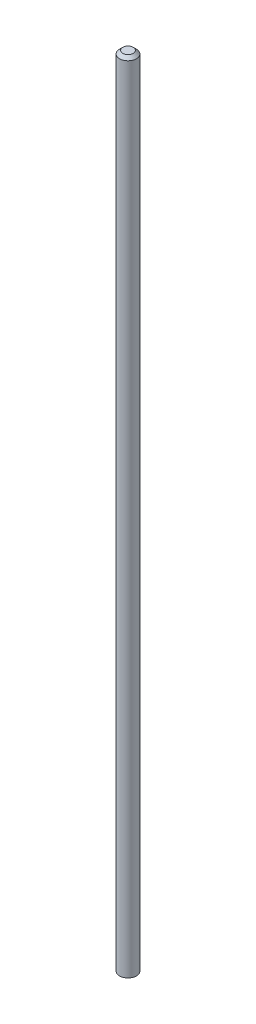
from build123d import *

# Parameters (mm, degrees)
SKETCH1_R           = 8
BOSS_EXTRUDE1_DEPTH = 759
CHAMFER1_SIZE       = 3


with BuildPart() as part:
    # Sketch1 → Boss-Extrude1 (new body)
    with BuildSketch(Plane(origin=(0, 0, 0), x_dir=(1, 0, 0), z_dir=(0, 1, 0))):
        with Locations(Location((0, 0, 0), (0, 0, 270))):
            Circle(SKETCH1_R)
    extrude(amount=BOSS_EXTRUDE1_DEPTH)

    # Chamfer1
    chamfer1_edges = [part.edges().sort_by_distance(p)[0] for p in [
        (0, 759, -8),
    ]]
    chamfer(chamfer1_edges, length=CHAMFER1_SIZE)


solid = part.part
